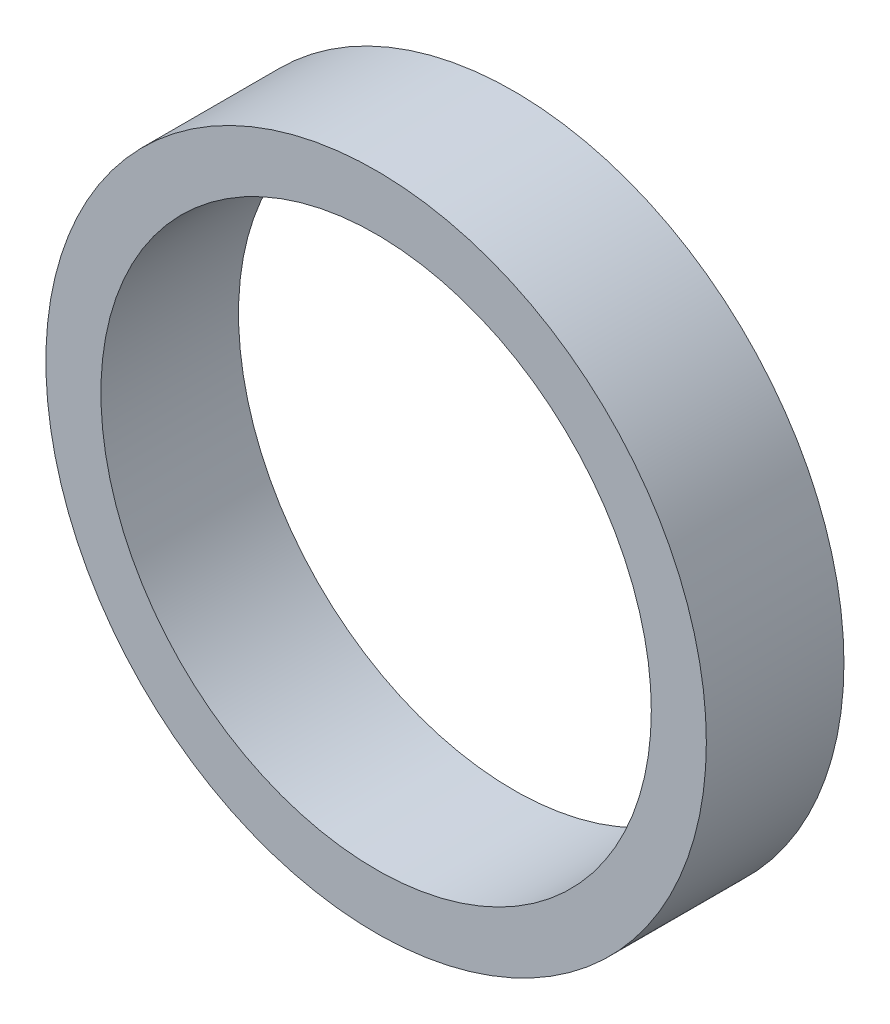
SolidWorks part; units mm, degrees
ref_plane "Front" through (0, 0, 0) normal (0, 0, 1) x (1, 0, 0)
ref_plane "Top" through (0, 0, 0) normal (0, 1, 0) x (1, 0, 0)
ref_plane "Right" through (0, 0, 0) normal (1, 0, 0) x (0, 0, -1)
sketch "草图2" plane through (0, 0, 0) normal (0, 0, 1) x (1, 0, 0)
  circle A0 centre (0, 0) radius 20
  circle A1 centre (0, 0) radius 24
extrude "凸台-拉伸1" add sketch "草图2" along normal blind 10
